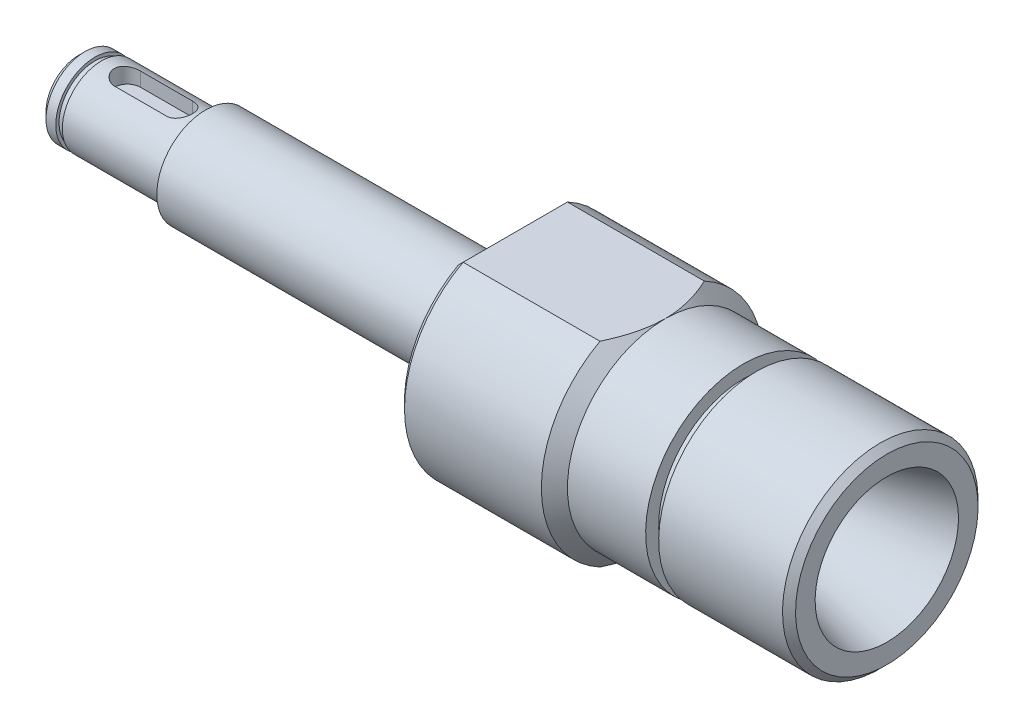
SolidWorks part; units mm, degrees
ref_plane "Front Plane" through (0, 0, 0) normal (0, 0, 1) x (1, 0, 0)
ref_plane "Top Plane" through (0, 0, 0) normal (0, 1, 0) x (1, 0, 0)
ref_plane "Right Plane" through (0, 0, 0) normal (1, 0, 0) x (0, 0, -1)
other "Configuration Table"
sketch "Sketch1" plane through (0, 0, 0) normal (0, 0, 1) x (1, 0, 0)
  line L0 (0, 0) -> (0, 6)
  line L1 (0, 6) -> (2.5, 6)
  line L2 (2.5, 6) -> (2.5, 5.5)
  line L3 (2.5, 5.5) -> (3.5, 5.5)
  line L4 (3.5, 5.5) -> (3.5, 6)
  line L5 (3.5, 6) -> (18.5, 6)
  line L6 (18.5, 6) -> (18.5, 5.5)
  line L7 (18.5, 5.5) -> (19.5, 5.5)
  line L8 (19.5, 5.5) -> (19.5, 7.5)
  line L9 (19.5, 7.5) -> (64, 7.5)
  line L10 (64, 7.5) -> (64, 6.5)
  line L11 (64, 6.5) -> (66, 6.5)
  line L12 (66, 6.5) -> (66, 17)
  line L13 (66, 17) -> (88, 17)
  line L14 (88, 17) -> (90, 15)
  line L15 (90, 15) -> (102, 15)
  line L16 (102, 15) -> (102, 13)
  line L17 (102, 13) -> (104, 13)
  line L18 (104, 13) -> (104, 15)
  line L19 (104, 15) -> (124, 15)
  line L20 (124, 15) -> (124, 0)
  line L21 (124, 0) -> (0, 0) construction
  line L22 (0, 0) -> (124, 0)
  dimension "D1" = 12
  dimension "D2" = 11
  dimension "D3" = 12
  dimension "D4" = 124
  dimension "D5" = 1
  dimension "D6" = 1
  dimension "D7" = 0.5
  dimension "D8" = 16
  dimension "D9" = 15
  dimension "D10" = 2
  dimension "D11" = 1
  dimension "D12" = 34
  dimension "D13" = 46.5
  dimension "D14" = 58
  dimension "D15" = 22
  dimension "D16" = 14
  dimension "D17" = 45
  dimension "D18" = 2
  dimension "D19" = 30
  dimension "D20" = 30
  dimension "D21" = 2
revolve "Revolve1" add sketch "Sketch1" angle 360 about L21
cosmetic thread "Cosmetic Thread1" parameters "D2"=26.211
sketch "Sketch3" plane through (0, 0, 0) normal (0, 1, 0) x (1, 0, 0)
  line L0 (15.5, 0) -> (7.5, 0) construction
  line L1 (15.5, -2) -> (7.5, -2)
  line L2 (15.5, 2) -> (7.5, 2)
  line L3 (3.5, 6) -> (3.5, -6) construction
  arc A0 (15.5, -2) -> (15.5, 2) centre (15.5, 0) ccw
  arc A1 (7.5, 2) -> (7.5, -2) centre (7.5, 0) ccw
  point P2 (11.5, 0)
  point P7 (5.5, 0)
  point P8 (17.5, 0)
  dimension "D1" = 12
  dimension "D2" = 2
  dimension "D3" = 4
extrude "Cut-Extrude1" cut sketch "Sketch3" along normal blind 10 from offset 3.5
sketch "Sketch6" plane through (66, 0, 0) normal (-1, 0, 0) x (0, 0, 1)
  line L0 (-8, 15) -> (8, 15)
  line L1 (-8, -15) -> (8, -15)
  line L2 (0, 0) -> (1.4574, 0) construction
  circle A0 centre (0, 0) radius 17 construction
  arc A1 (-8, -15) -> (8, -15) centre (0, 0) ccw
  arc A2 (8, 15) -> (-8, 15) centre (0, 0) ccw
  dimension "D1" = 30
extrude "Cut-Extrude2" cut sketch "Sketch6" against normal up to next
chamfer "Chamfer1" distance 1 angle 45 6 edges at (124, 15, 0) (66, -15, 0) (66, 0, -17) (66, 0, 17) (66, 15, 0) (0, 6, 0)
sketch "Sketch7" plane through (0, 0, 0) normal (0, 0, 1) x (1, 0, 0)
  line L0 (124, 11) -> (108, 6.7128)
  line L1 (124, -14) -> (124, 14) construction
  line L2 (108, 6.7128) -> (108, 9.5)
  line L3 (108, 9.5) -> (103, 9.5)
  line L4 (103, 9.5) -> (103, 9)
  line L5 (103, 9) -> (97, 9)
  line L6 (97, 9) -> (97, 9.5)
  line L7 (97, 9.5) -> (92, 9.5)
  line L8 (92, 9.5) -> (92, 7)
  line L10 (92, 7) -> (76, 7)
  line L11 (76, 7) -> (71.9585, 0)
  line L12 (71.9585, 0) -> (124, 0) construction
  line L13 (124, 0) -> (124, 11)
  line L14 (71.9585, 0) -> (124, 0)
  dimension "D1" = 15
  dimension "D2" = 22
  dimension "D3" = 5
  dimension "D4" = 6
  dimension "D5" = 5
  dimension "D6" = 19
  dimension "D7" = 19
  dimension "D8" = 32
  dimension "D9" = 18
  dimension "D10" = 48
  dimension "D11" = 14
  dimension "D12" = 60
revolve "Cut-Revolve1" cut sketch "Sketch7" angle 360 about L12
chamfer "Chamfer2" distance 1 angle 45 1 edges at (92, -7, 0)
